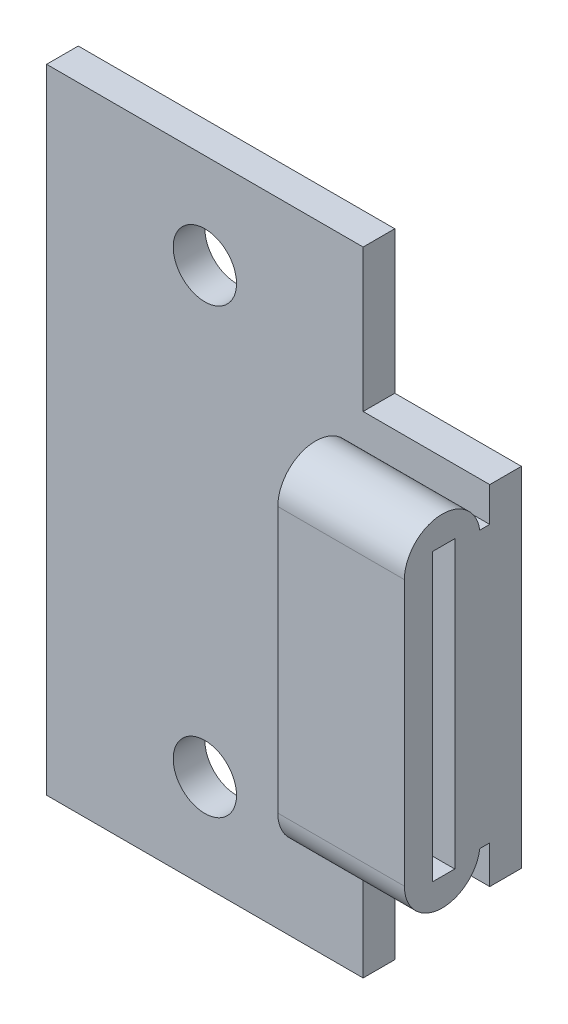
from build123d import *

# Parameters (mm, degrees)
SKETCH1_R           = 1
BOSS_EXTRUDE1_DEPTH = 1
SKETCH2_W           = 4
SKETCH2_H           = 11
BOSS_EXTRUDE2_DEPTH = 3
SKETCH3_W           = 3
SKETCH3_H           = 11
CUT_EXTRUDE1_DEPTH  = 10
SKETCH4_W           = 0.703476056
SKETCH4_H           = 9.036961638
CUT_EXTRUDE2_DEPTH  = 3
SKETCH5_W           = 0.607326988
SKETCH5_H           = 8.712280381
BOSS_EXTRUDE3_DEPTH = 4


with BuildPart() as part:
    # Sketch1 → Boss-Extrude1 (new body)
    with BuildSketch(Plane.XY):
        Polygon((-5, 10), (5, 10), (5, 5.5), (9, 5.5), (9, -5.5), (5, -5.5), (5, -10), (-5, -10), align=None)
        with Locations((0, 7)):
            Circle(SKETCH1_R, mode=Mode.SUBTRACT)
        with Locations((0, -7)):
            Circle(SKETCH1_R, mode=Mode.SUBTRACT)
    extrude(amount=BOSS_EXTRUDE1_DEPTH)

    # Sketch2 → Boss-Extrude2 (add)
    with BuildSketch(Plane.XY.offset(1)):
        with Locations((7, 0)):
            Rectangle(SKETCH2_W, SKETCH2_H)
    extrude(amount=BOSS_EXTRUDE2_DEPTH)

    # Sketch3 → Cut-Extrude1 (cut)
    with BuildSketch(Plane(origin=(9, 0, 0), x_dir=(0, 0, -1), z_dir=(1, 0, 0))):
        with Locations((-2.5, 0)):
            Rectangle(SKETCH3_W, SKETCH3_H)
        with BuildLine():
            Line((-1.303663494, 4.247913105), (-1.303663494, -4.13968602))
            ThreePointArc((-1.303663494, -4.13968602), (-2.5, -5.336022526), (-3.696336506, -4.13968602))
            Line((-3.696336506, -4.13968602), (-3.696336506, 4.247913105))
            ThreePointArc((-3.696336506, 4.247913105), (-2.5, 5.444249611), (-1.303663494, 4.247913105))
        make_face(mode=Mode.SUBTRACT)
    extrude(amount=-CUT_EXTRUDE1_DEPTH, mode=Mode.SUBTRACT)


with BuildPart() as cut_extrude1_piece_1:
    # of the separate pieces the step leaves, piece 1, a body of its own (cut_extrude1_pieces)
    add(part.part.solids().sort_by_distance((-5, 10, 0))[0])



with BuildPart() as cut_extrude1_piece_2:
    # of the separate pieces the step leaves, piece 2, a body of its own (cut_extrude1_pieces)
    add(part.part.solids().sort_by_distance((9, 4.247913105, 3.696336506))[0])

    # Sketch4 → Cut-Extrude2 (cut)
    with BuildSketch(Plane(origin=(9, 0, 0), x_dir=(0, 0, -1), z_dir=(1, 0, 0))):
        with Locations((-2.456945609, 0.054113543)):
            Rectangle(SKETCH4_W, SKETCH4_H)
    extrude(amount=-CUT_EXTRUDE2_DEPTH, mode=Mode.SUBTRACT)


with BuildPart() as cut_extrude1_piece_1_1:
    add(cut_extrude1_piece_1.part)

    add(cut_extrude1_piece_2.part)  # Boss-Extrude3 merges Cut-Extrude1 piece 2
    # Sketch5 → Boss-Extrude3 (add)
    with BuildSketch(Plane(origin=(9, 0, 0), x_dir=(0, 0, -1), z_dir=(1, 0, 0))):
        with Locations((-1.303663494, 0.054113543)):
            Rectangle(SKETCH5_W, SKETCH5_H)
    extrude(amount=-BOSS_EXTRUDE3_DEPTH)


solid = cut_extrude1_piece_1_1.part
